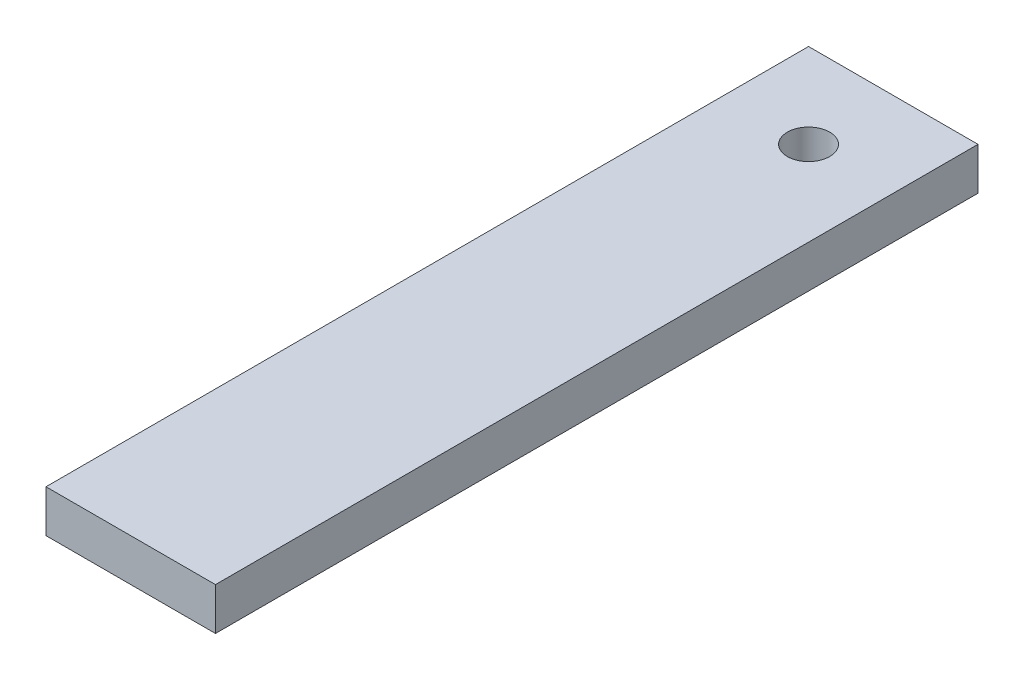
SolidWorks part; units mm, degrees
ref_plane "Front Plane" through (0, 0, 0) normal (0, 0, 1) x (1, 0, 0)
ref_plane "Top Plane" through (0, 0, 0) normal (0, 1, 0) x (1, 0, 0)
ref_plane "Right Plane" through (0, 0, 0) normal (1, 0, 0) x (0, 0, -1)
sketch "Sketch1" plane through (0, 0, 0) normal (0, 1, 0) x (1, 0, 0)
  line L1 (-10, -45) -> (10, -45)
  line L2 (-10, -45) -> (-10, 45)
  line L3 (-10, 45) -> (10, 45)
  line L4 (10, -45) -> (10, 45)
  line L5 (-10, -45) -> (10, 45) construction
  line L6 (-10, 45) -> (10, -45) construction
  circle A0 centre (0, 35) radius 2.5
  point P0 (0, 0)
  dimension "D3" = 5
  dimension "D4" = 10
  dimension "D1" = 20
  dimension "D2" = 90
extrude "Boss-Extrude1" add sketch "Sketch1" along normal blind 5
